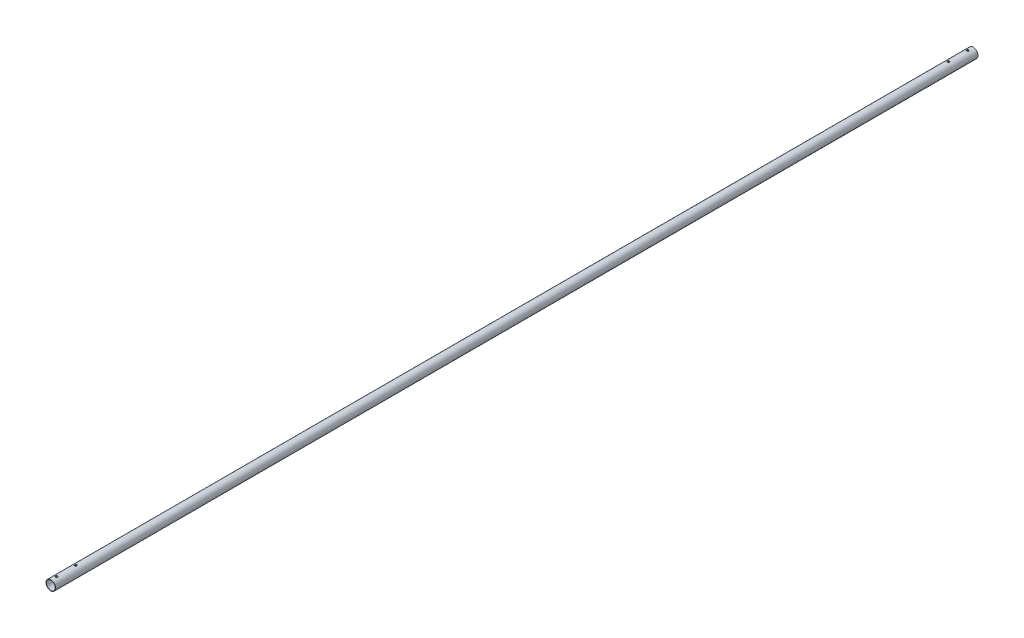
from build123d import *

# Parameters (mm, degrees)
SKETCH_2_R               = 7
SKETCH_2_R_2             = 6.5
EXTRUDE_2_DEPTH          = 1336
CUT_EXTRUDE_1_DEPTH      = 1337.036676143
CUT_EXTRUDE_1_DEPTH_BACK = 1337.036676143
SKETCH_3_R               = 1.55


with BuildPart() as part:
    # 草图2 → 凸台-拉伸2 (new body)
    with BuildSketch(Plane.XY):
        with Locations(Location((0, 0, 0), (0, 0, 180))):
            Circle(SKETCH_2_R)
        with Locations(Location((0, 0, 0), (0, 0, 180))):
            Circle(SKETCH_2_R_2, mode=Mode.SUBTRACT)
    extrude(amount=EXTRUDE_2_DEPTH)

    # 草图3 → 切除-拉伸1 (cut, two sides: drawn at the far end of the back side and taken through both)
    with BuildSketch(Plane(origin=(0, 0, 0), x_dir=(1, 0, 0), z_dir=(0, 1, 0)).offset(-CUT_EXTRUDE_1_DEPTH_BACK)):
        with Locations(Location((0, -8, 0), (0, 0, 270))):
            Circle(SKETCH_3_R)
        with Locations(Location((0, -36, 0), (0, 0, 270))):
            Circle(SKETCH_3_R)
        with Locations(Location((0, -1328, 0), (0, 0, 270))):
            Circle(SKETCH_3_R)
        with Locations(Location((0, -1300, 0), (0, 0, 270))):
            Circle(SKETCH_3_R)
    extrude(amount=CUT_EXTRUDE_1_DEPTH + CUT_EXTRUDE_1_DEPTH_BACK, mode=Mode.SUBTRACT)


solid = part.part
